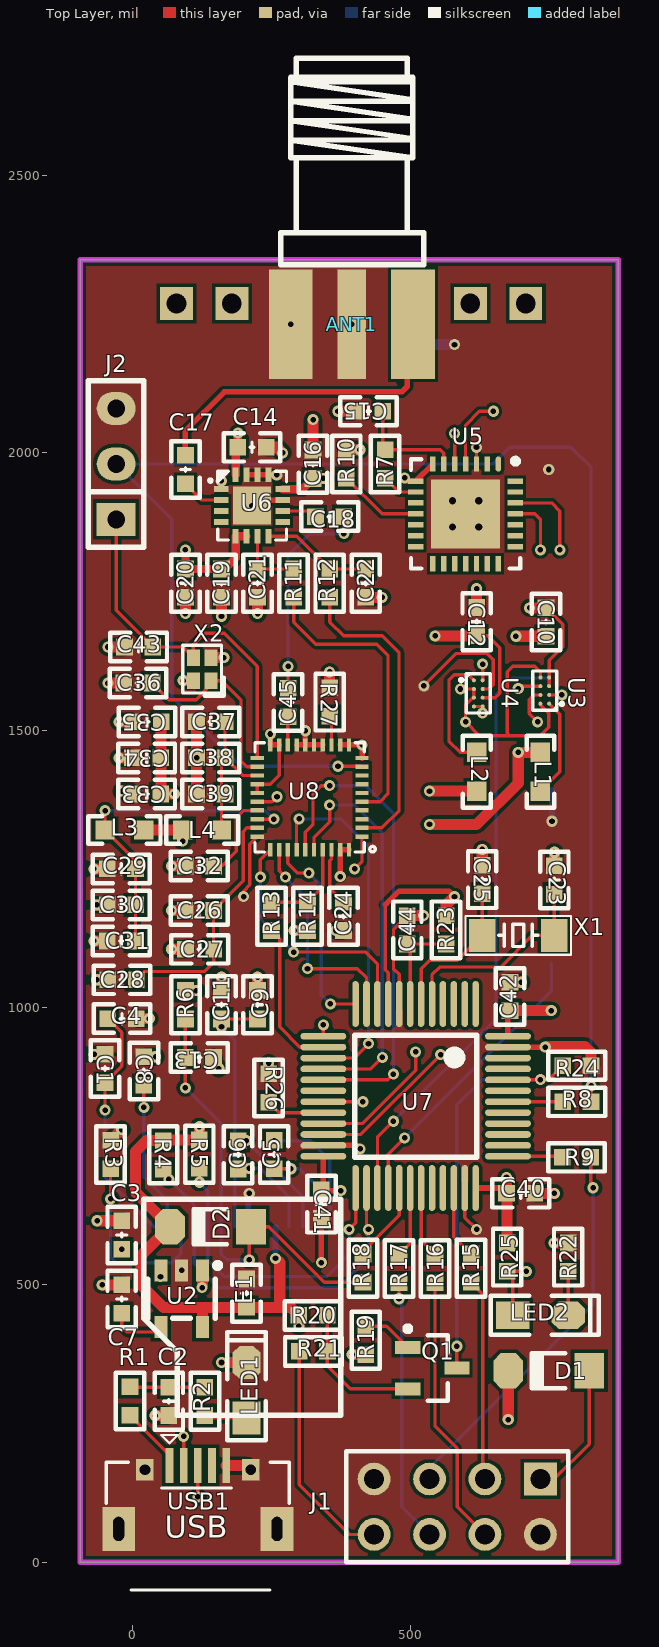
[diagram p0: Top Layer view]
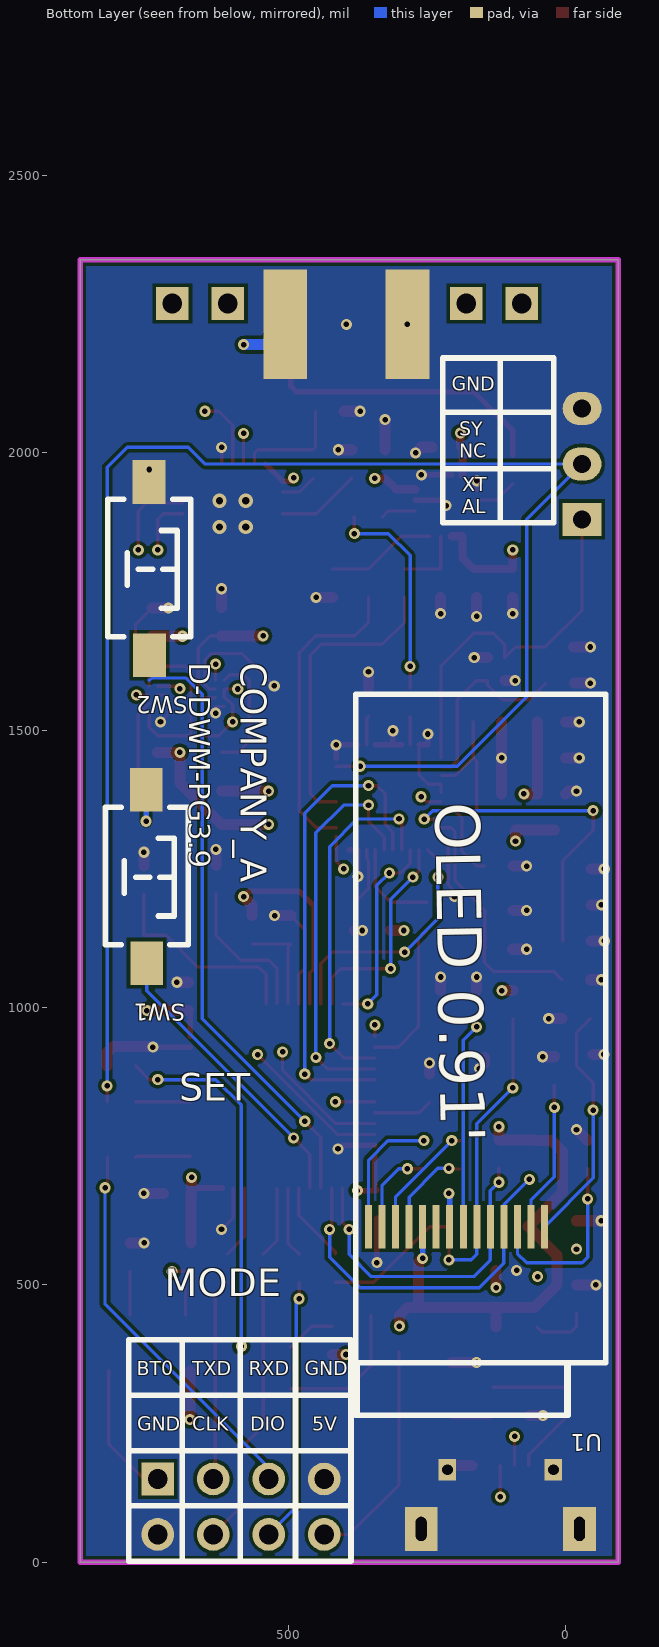
[diagram p1: Bottom Layer view, seen from below]
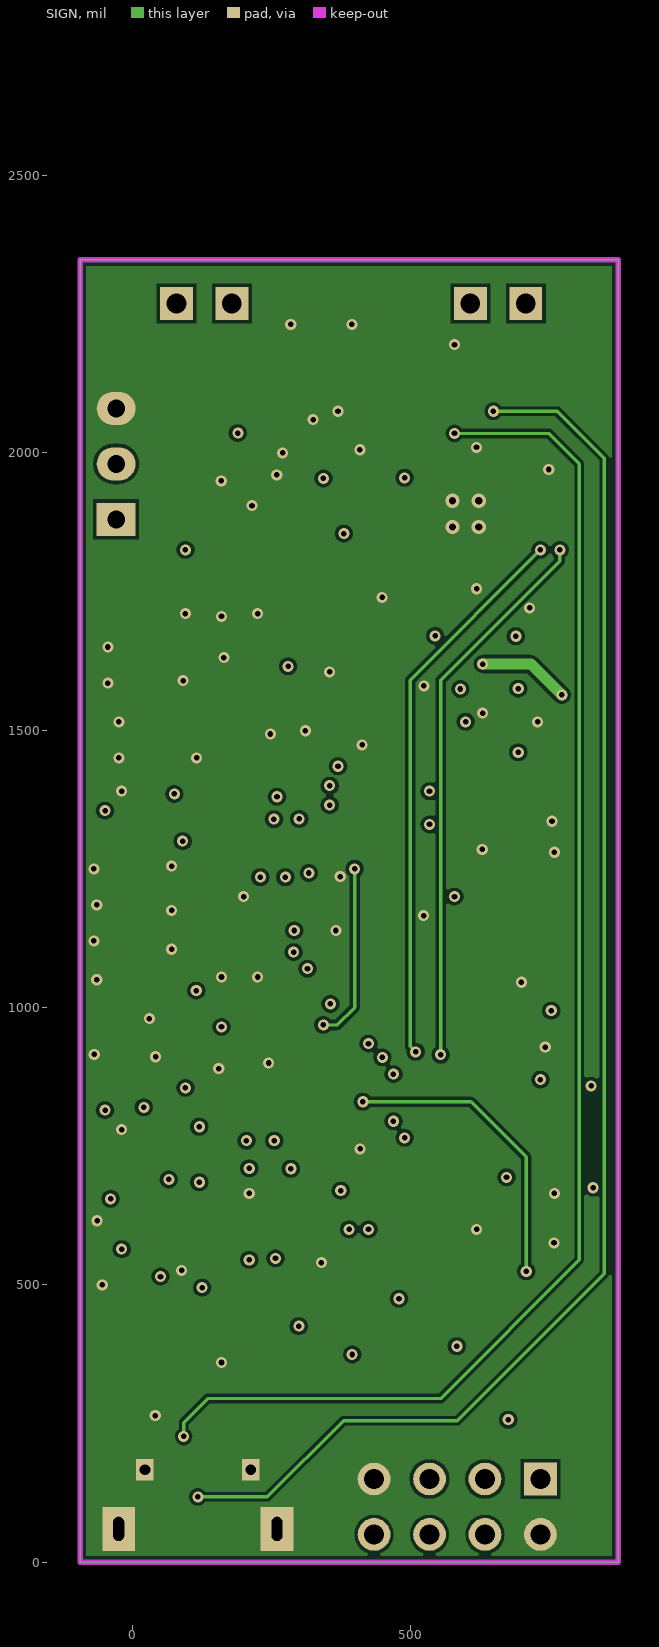
[diagram p2: SIGN]
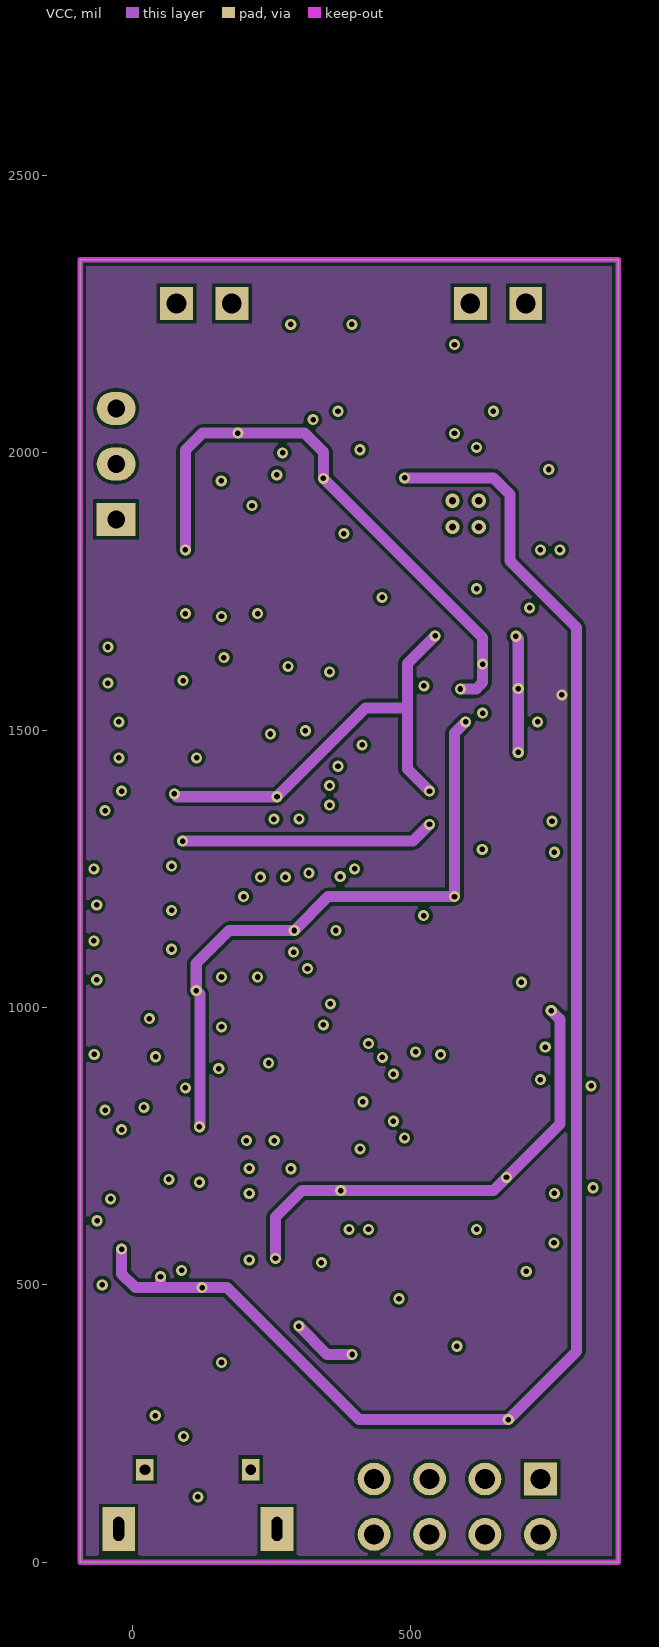
[diagram p3: VCC]
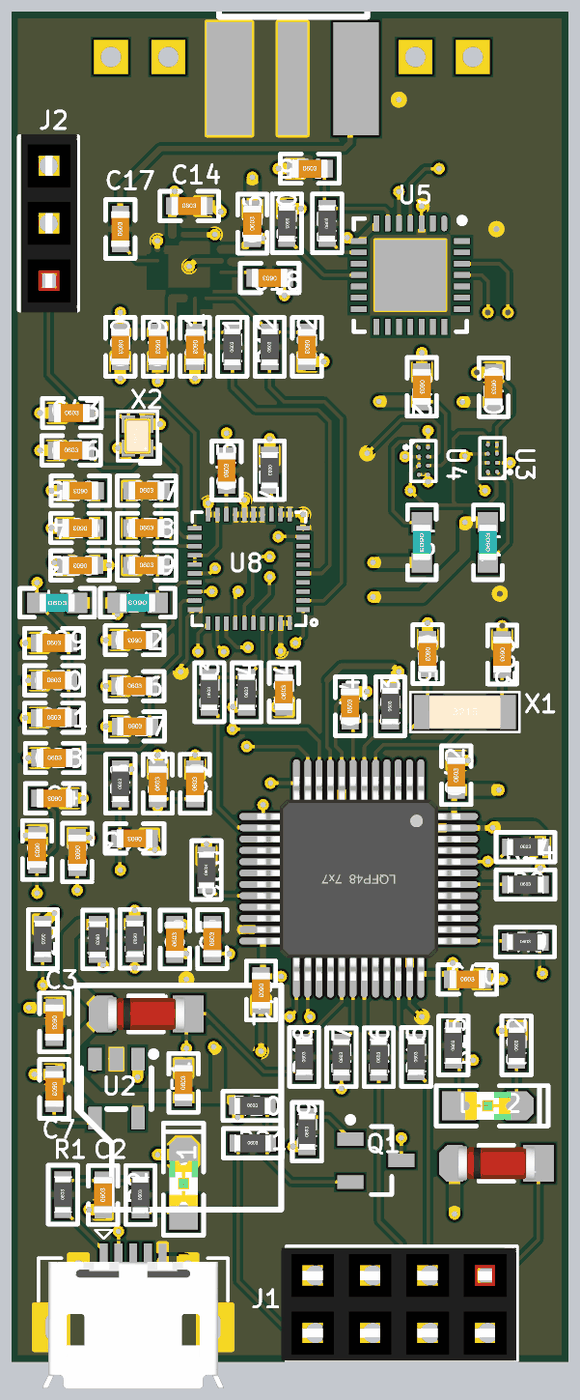
[diagram p4: 3D render of the assembled board from above, using the file's embedded part models]
# Altium PCB MISC85928.PcbDoc
Units mil, origin at the board's own origin, x right, y up, seen from the top; angles counter-clockwise.
Board outline 970 x 2348 mil, 4 copper layers (Top Layer, SIGN, VCC, Bottom Layer); 98 components, 80 nets, 373 pads, 153 vias.

## Layer stack, top to bottom (the 12.6 mil dielectric is the usual default, probably not edited)
Top Solder: solder mask 0.4, Solder Resist, Dk 3.5
Top Layer: signal copper 1.4
Dielectric1: core 12.6, FR-4, Dk 4.8
SIGN: signal copper 1.4
Dielectric3: core 12.6, FR-4, Dk 4.8
VCC: signal copper 1.4
Dielectric2: prepreg 12.6, FR-4, Dk 4.8
Bottom Layer: signal copper 1.4
Bottom Solder: solder mask 0.4, Solder Resist, Dk 3.5

## Board outline
-95,0 875,0 875,2348 -95,2348

## Design rules (kind name [scope] priority, off if disabled: settings)
Clearance [All] p1: gap=6 ignorepadtopadclearanceinfootprint=FALSE
MinimumSolderMaskSliver [All] p1: minsoldermaskwidth=0
PlaneConnect [All] p1: planeconnectstyle=Direct reliefexpansion=20 reliefentries=4 reliefconductorwidth=10 reliefairgap=10
PolygonConnect [All] p1: connectstyle=Direct reliefconductorwidth=10 reliefentries=4 polygonreliefangle="90 Angle" airgapwidth=10
RoutingVias [All] p1: holewidth=11.81 width=17.72 viastyle="Through Hole" minholewidth=11.81 minwidth=17.72 maxholewidth=11.81 maxwidth=17.72
SilkToSilkClearance [All] p1: silktosilkclearance=0
SilkToSolderMaskClearance SilkscreenOverComponentPads [IsPad] p1: minsilkscreentomaskgap=0 clearancetoexposedcopper=TRUE
SolderMaskExpansion [All] p1: expansion=4 istentingtop=FALSE
Width [All] p1: maxlimit=20 minlimit=5 preferedwidth=5
26 further rules are at their usual default settings.

## Components (designator, comment, footprint, x,y, rotation, side; value= is the part's Value field where it differs from the comment)
ANT1 "Partron" ÌìÏß×ù5p 395,2425 r90 top locked
C1 "100nF" "C 0603_L" -50,890 r270 top
C2 "100nF" "C 0603_L" 65,290 r90 top
C3 "10uF" "C 0603_L" -20,590 r270 top
C4 "4.7uF" "C 0603_L" -19.41,980 r180 top
C5 "1uF" "C 0603_L" 255,735 r90 top
C6 "1uF" "C 0603_L" 190,734.41 r90 top
C7 "100nF" "C 0603_L" -20,474.41 r270 top
C8 "2.2uF" "C 0603_L" 20,885.59 r270 top
C9 "100nF" "C 0603_L" 225,1005 r90 top
C10 "10uF" "C 0603_L" 745,1695 r270 top
C11 "4.7uF" "C 0603_L" 160,1005 r90 top
C12 "10uF" "C 0603_L" 620,1695.59 r270 top
C13 "4.7uF" "C 0603_L" 120,910 r180 top
C14 "1nF" "C 0603_L" 215,2010 r0 top
C15 "4.7uF" "C 0603_L" 425,2075 r0 top
C16 "1nF" "C 0603_L" 325,1979.41 r90 top
C17 "100pF" "C 0603_L" 95,1970 r90 top
C18 "100pF" "C 0603_L" 355,1885 r180 top
C19 "1nF" "C 0603_L" 160,1765 r270 top
C20 "1nF" "C 0603_L" 95,1765 r270 top
C21 "1nF" "C 0603_L" 225,1765 r270 top
C22 "1nF" "C 0603_L" 420,1765 r270 top
C23 "20pF" "C 0603_L" 760,1230 r270 top
C24 "100nF" "C 0603_L" 380,1164.41 r90 top
C25 "20pF" "C 0603_L" 630,1230.59 r270 top
C26 "2pF" "C 0603_L" 120,1175 r0 top
C27 "100nF" "C 0603_L" 120.59,1105 r0 top
C28 "22uF" "C 0603_L" -19.41,1050 r0 top
C29 "4.7nF" "C 0603_L" -20.59,1250 r0 top
C30 "100nF" "C 0603_L" -20.59,1185 r0 top
C31 "10uF" "C 0603_L" -20.59,1120 r0 top
C32 "220nF" "C 0603_L" 120,1255 r180 top
C33 "4.7nF" "C 0603_L" 25,1385 r180 top
C34 "100nF" "C 0603_L" 25,1450 r180 top
C35 "10uF" "C 0603_L" 25.59,1515 r180 top
C36 "8pF" "C 0603_L" 9.41,1585 r0 top
C37 "4.7nF" "C 0603_L" 140.59,1515 r0 top
C38 "100nF" "C 0603_L" 140.59,1450 r0 top
C39 "10uF" "C 0603_L" 140.59,1385 r0 top
C40 "100nF" "C 0603_L" 699.41,665 r0 top
C41 "100nF" "C 0603_L" 340,645.59 r270 top
C42 "100nF" "C 0603_L" 680,1020 r90 top
C43 "8pF" "C 0603_L" 10.59,1650 r0 top
C44 "100nF" "C 0603_L" 495,1140 r90 top
C45 "2pF" "C 0603_L" 280,1550 r90 top
D1 "SS34" "MINI_MELF (LL34)" 750,345 r180 top
D2 "1N4148" "MINI_MELF (LL34)" 140,605 r180 top
E1 "22uF/6.3V" "C 0603_L" 205,485 r90 top
J1 "Female HDR2X4" Fe-HDR2X4/2.54-S 735,150 r180 top locked
J2 "Female HDR1X3" Fe-HDR1X3/2.54-S -30,1880 r180 top
L1 "Inductor Iron" "L 0603" 735,1425 r90 top
L2 "Inductor Iron" "L 0603" 620,1425 r270 top
L3 "600R" "L 0603" -15,1320 r0 top
L4 "600R" "L 0603" 125,1320 r180 top
LED1 "Red" "LED 0805G" 205,310 r90 top
LED2 "Red" "LED 0805G" 735,445 r0 top
Q1 "S9012" SOT-23B_N 540,350 r0 top
R1 "B5R" "R 0603_L" -5,290.59 r90 top
R2 "470R" "R 0603_L" 130,290 r90 top
R3 "4.7K" "R 0603_L" -40,735 r270 top
R4 "4.7K" "R 0603_L" 55,734.41 r270 top
R5 "4.7K" "R 0603_L" 120,735.59 r270 top
R6 "4.7K" "R 0603_L" 95,1005 r90 top
R7 "4.7K" "R 0603_L" 455,1980 r90 top
R8 "0R" "R 0603_L" 800.59,830 r0 top
R9 "22R" "R 0603_L" 800,730 r0 top
R10 "10K" "R 0603_L" 385,1980 r270 top
R11 "0R" "R 0603_L" 290,1765 r90 top
R12 "0R" "R 0603_L" 355,1765 r90 top
R13 "100R" "R 0603_L" 250,1164.41 r90 top
R14 "DNF" "R 0603_L" 315,1164.41 r90 top
R15 "22R" "R 0603_L" 610,530 r90 top
R16 "22R" "R 0603_L" 545,529.41 r90 top
R17 "22R" "R 0603_L" 480,529.41 r90 top
R18 "22R" "R 0603_L" 415,530 r90 top
R19 "1K" "R 0603_L" 420,400 r90 top
R20 "1K" "R 0603_L" 325,445 r0 top
R21 "1K" "R 0603_L" 325.59,380 r0 top
R22 "470R" "R 0603_L" 785,550 r90 top
R23 "1K" "R 0603_L" 565,1140 r90 top
R24 "10K" "R 0603_L" 800.59,895 r0 top
R25 "10K" "R 0603_L" 675,550 r90 top
R26 "10K" "R 0603_L" 245,855 r90 top
R27 "49R9" "R 0603_L" 355,1550.59 r270 top
SW1 "3x6x5" "TSW SMD-3*6*2.5" 755,1235 r270 bottom
SW2 "3x6x5" "TSW SMD-3*6*2.5" 750,1790 r270 bottom
U1 "0.91-OLED" OLED0.91 152.67,914.72 r270 bottom locked
U2 "TPS736" SOT-23-5_L3.0-W1.7-P0.95-LS2.8-BR 90,475 r90 top
U3 "TPS62743YFPR" DSBGA-8_L1.6-W0.9-R2-C4-P0.40-BL 747.35,1571.38 r90 top
U4 "TPS62743YFPR" DSBGA-8_L1.6-W0.9-R2-C4-P0.40-BL 618.4,1566.38 r270 top
U5 "CP2102" CP2102 600,1890 r270 top
U6 "SW8112Q" QFN-16_L3.0-W3.0-P0.50-BL-EP1.7 16373.05,20632.78 r270 top
U7 "STM32F103C8T6" "LQFP48 7X7" 510,840 r180 top
U8 "DW3210" DW3210 325,1375 r180 top
USB1 "USB-5P" USB-MICRO_A 117.28,60 r0 top locked
X1 "16MHz" "OSC 3215-2P" 695,1130 r0 top
X2 "38.4MHZ" "OSC 1612-4P" 125,1610 r90 top

## Footprints (in the part's own frame and the unit in brackets; to place one, negate y for a bottom-side part, rotate by r counter-clockwise, add the part's x,y. Pads: shape width x height; smd on the part's side, far side on the other; paste and mask are expansions set on the pad)
"C 0603_L" [mil] "ÎÞ¼«ÐÔÌùÆ¬µçÈÝ"
  rect 30x30 smd: 1(-25.59,0) 2(25.59,0)
  silkscreen extent -51,-26 51,26, body extent -31,-16 31,16, height 32
CP2102 [mm]
  oval 0.7x0.25 smd paste+0 mask+0.051: 1(-2.28,1.5)
  rect 0.7x0.25 smd paste+0 mask+0.051: 2(-2.28,1) 3(-2.28,0.5) 4(-2.28,0) 5(-2.28,-0.5) 6(-2.28,-1) 7(-2.28,-1.5) 15(2.28,-1.5) 16(2.28,-1) 17(2.28,-0.5) 18(2.28,0) 19(2.28,0.5) 20(2.28,1) 21(2.28,1.5)
  rect 0.25x0.7 smd paste+0 mask+0.051: 8(-1.5,-2.28) 9(-1,-2.28) 10(-0.5,-2.28) 11(0,-2.28) 12(0.5,-2.28) 13(1,-2.28) 14(1.5,-2.28) 22(1.5,2.28) 23(1,2.28) 24(0.5,2.28) 25(0,2.28) 26(-0.5,2.28) 27(-1,2.28) 28(-1.5,2.28)
  rect 3.15x3.15 smd paste+0 mask+0.051: 29(0,0)
  silkscreen extent -2.54,-2.5 2.5,2.5
DSBGA-8_L1.6-W0.9-R2-C4-P0.40-BL [mm]
  round 0.184 smd paste+0 mask+0.051: A1(-0.6,-0.086) A2(-0.6,0.314) B1(-0.2,-0.086) B2(-0.2,0.314) C1(0.2,-0.086) C2(0.2,0.314) D1(0.6,-0.086) D2(0.6,0.314)
  silkscreen extent -0.9,-0.74 0.9,0.66
DW3210 [mm]
  rect 0.6x0.2 smd paste+0 mask+0.051: 1(-2.246,1.7) 2(-2.246,1.3) 3(-2.246,0.9) 4(-2.246,0.5) 5(-2.246,0.1) 6(-2.246,-0.3) 7(-2.246,-0.7) 8(-2.246,-1.1) 9(-2.246,-1.5) 10(-2.246,-1.9) 21(2.554,-1.9) 22(2.554,-1.5) 23(2.554,-1.1) 24(2.554,-0.7) 25(2.554,-0.3) 26(2.554,0.1) 27(2.554,0.5) 28(2.554,0.9) 29(2.554,1.3) 30(2.554,1.7)
  rect 0.2x0.6 smd paste+0 mask+0.051: 11(-1.646,-2.5) 12(-1.246,-2.5) 13(-0.846,-2.5) 14(-0.446,-2.5) 15(-0.046,-2.5) 16(0.354,-2.5) 17(0.754,-2.5) 18(1.154,-2.5) 19(1.554,-2.5) 20(1.954,-2.5) 31(1.954,2.3) 32(1.554,2.3) 33(1.154,2.3) 34(0.754,2.3) 35(0.354,2.3) 36(-0.046,2.3) 37(-0.446,2.3) 38(-0.846,2.3) 39(-1.246,2.3) 40(-1.646,2.3)
  silkscreen extent -2.85,-2.6 2.65,2.4
Fe-HDR1X3/2.54-S [mil]
  rect 70x60 hole 32: 1(0,0)
  oval 70x60 hole 32: 2(0,-100) 3(0,-200)
  silkscreen extent -50,-250 50,50, body extent -50,-255 48,55, height 335
Fe-HDR2X4/2.54-S [mm] "Connector; Header; 4x2 Position"
  rect 1.5x1.5 hole 0.9: 1(0,0)
  round 1.5 hole 0.9: 2(0,2.54) 3(2.54,0) 4(2.54,2.54) 5(5.08,0) 6(5.08,2.54) 7(7.62,0) 8(7.62,2.54)
  silkscreen extent -1.27,-1.27 8.89,3.81, body extent -1.27,-1.23 9.14,3.77, height 8.5
"L 0603" [mil] "Ð¡¹¦ÂÊÌùÆ¬µç¸Ð"
  rect 35x35 smd: 1(-35,0) 2(35,0)
  silkscreen extent -65,-25 65,25, body extent -31,-16 31,16, height 31
"LED 0805G" [mil] "ÂÌÉ«0805LED"
  rect 60x50 smd: 1(-50,0)
  oct 60x50 smd: 2(50,0)
  silkscreen extent -90,-35 105,35, body extent -39,-25 39,25, height 32
"LQFP48 7X7" [mm]
  oval 0.3x2.1 smd: 1(-2.75,-4.227) 2(-2.25,-4.227) 3(-1.75,-4.227) 4(-1.25,-4.227) 5(-0.75,-4.227) 6(-0.25,-4.227) 7(0.25,-4.227) 8(0.75,-4.227) 9(1.25,-4.227) 10(1.75,-4.227) 11(2.25,-4.227) 12(2.75,-4.227) 25(2.75,4.202) 26(2.25,4.202) 27(1.75,4.202) 28(1.25,4.202) 29(0.75,4.202) 30(0.25,4.202) 31(-0.25,4.202) 32(-0.75,4.202) 33(-1.25,4.202) 34(-1.75,4.202) 35(-2.25,4.202) 36(-2.75,4.202)
  oval 2.1x0.3 smd: 13(4.227,-2.75) 14(4.227,-2.25) 15(4.227,-1.75) 16(4.227,-1.25) 17(4.227,-0.75) 18(4.227,-0.25) 19(4.227,0.25) 20(4.227,0.75) 21(4.227,1.25) 22(4.227,1.75) 23(4.227,2.25) 24(4.227,2.75) 37(-4.227,2.75) 38(-4.227,2.25) 39(-4.227,1.75) 40(-4.227,1.25) 41(-4.227,0.75) 42(-4.227,0.25) 43(-4.227,-0.25) 44(-4.227,-0.75) 45(-4.227,-1.25) 46(-4.227,-1.75) 47(-4.227,-2.25) 48(-4.227,-2.75)
  silkscreen extent -2.79,-2.79 2.79,2.79, body extent -4.51,-4.5 4.5,4.5, height 1.45
"MINI_MELF (LL34)" [mm] "1.5*3.4mm(Ö±¾¶£¬½Å¾à£©"
  rect 1.37x1.62 smd: 1(-1.855,0)
  oct 1.37x1.62 smd: 2(1.855,0)
  silkscreen extent -0.76,-0.8 0.78,0.8, body extent -1.7,-0.75 1.7,0.75, height 1.5
OLED0.91 [mm]
  rect 2x0.32 smd paste+0 mask+0.051: 1(7.867,-5.139) 2(7.867,-4.519) 3(7.867,-3.899) 4(7.867,-3.279) 5(7.867,-2.659) 6(7.867,-2.039) 7(7.867,-1.419) 8(7.867,-0.799) 9(7.867,-0.179) 10(7.867,0.441) 11(7.867,1.061) 12(7.867,1.681) 13(7.867,2.301) 14(7.867,2.921)
  silkscreen extent -16.51,-5.72 16.51,5.71
"OSC 1612-4P" [mm] "1.6*1.2*0.35mm£¨³¤¿í¸ß£©"
  rect 0.75x0.6 smd: 1(-0.525,-0.4) 2(0.525,-0.4) 3(0.525,0.4) 4(-0.525,0.4)
  silkscreen extent -1.22,-0.99 1.09,0.89, body extent -0.8,-0.6 0.8,0.6, height 0.35
"OSC 3215-2P" [mm] "3.2*1.5*0.6mm(³¤¿í¸ß)"
  rect 1.2x1.5 smd: 1(-1.65,0) 2(1.65,0)
  silkscreen extent -2.41,-0.89 2.41,0.89, body extent -1.6,-0.75 1.6,0.75, height 0.61
QFN-16_L3.0-W3.0-P0.50-BL-EP1.7 [mm]
  rect 0.28x0.665 smd paste-100 mask+0.051: 1(474.935,-411.822) 2(475.435,-411.822) 3(475.936,-411.822) 4(476.436,-411.822) 9(476.436,-409.007) 10(475.936,-409.007) 11(475.435,-409.007) 12(474.935,-409.007)
  rect 0.665x0.28 smd paste-100 mask+0.051: 5(477.093,-411.165) 6(477.093,-410.665) 7(477.093,-410.165) 8(477.093,-409.665) 13(474.278,-409.665) 14(474.278,-410.165) 15(474.278,-410.665) 16(474.278,-411.165)
  rect 1.75x1.75 smd paste-100 mask+0.051: 17(475.685,-410.415)
  silkscreen extent 474.11,-412.39 477.26,-408.84
"R 0603_L" [mil] "1/10WÌùÆ¬µç×è"
  rect 30x30 smd: 1(-25.59,0) 2(25.59,0)
  silkscreen extent -51,-26 51,26, body extent -31,-16 32,16, height 16
SOT-23-5_L3.0-W1.7-P0.95-LS2.8-BR [mm]
  rect 1x0.6 smd paste+0 mask+0.051: 1(1.3,-0.899) 2(1.3,0.051) 3(1.3,1) 4(-1.3,1) 5(-1.3,-0.899)
  silkscreen extent -0.9,-1.73 1.65,1.6
SOT-23B_N [mm] "SOT23, 3-Leads, Body 2.9x1.3mm, Pitch 0.95mm, Lead Span 2.4mm, IPC Medium Density"
  rect 1.15x0.6 smd: 1(-1.125,0.95) 2(-1.125,-0.95) 3(1.125,0)
  silkscreen extent -1.25,-1.5 0.7,1.92, body extent -0.7,-1.5 0.7,1.5, height 1.14
"TSW SMD-3*6*2.5" [mm] "3*6*2.5mm"
  rect 2x1.5 smd: 1(-3.996,-0.02) 2(3.937,0)
  silkscreen extent -3.21,-1.9 3.09,1.9, body extent -4,-1.88 4,1.62, height 2.59
USB-MICRO_A [mm] "microÐÍUSB £¬5.7*7.8*2.5mm"
  rect 0.35x1.6 smd: 1(-1.3,2.9) 2(-0.65,2.9) 3(0,2.9) 4(0.65,2.9) 5(1.3,2.9)
  rect 1.5x2 hole 0.5 slot 1.1 at 90 deg: 5(-3.625,0) 5(3.625,0)
  rect 0.8x1 hole 0.5: 5(-2.425,2.71) 5(2.425,2.71)
  silkscreen extent -4.19,-2.79 4.19,4.3, body extent -4,-2.71 4,2.89, height 2.8
ÌìÏß×ù5p [mm]
  rect 5x2 smd paste+0 mask+0.102: 1(-4.91,-2.8) 2(-4.91,2.8)
  rect 5x2 smd far side paste+0 mask+0.102: 3(-4.91,2.8) 4(-4.91,-2.8)
  rect 5x1.3 smd paste+0 mask+0.102: 5(-4.91,0)
  silkscreen extent -2.18,-3.3 7.28,3.25

## Part data
C1 C2 C3 C4 C5 C6 C7 C8 C9 C10 C11 C12 C13 C14 C15 C16 C17 C18 C19 C20 C21 C22 C23 C24 C25 C26 C27 C28 C29 C30 C31 C32 C33 C34 C35 C36 C37 C38 C39 C40 C41 C42 C43 C44 C45: library part C, "Chip capacitor"
D1: library part 1N4148, "Switching diode"
D2: "Switching diode"
E1: library part CT, "Chip tantalum capacitor"
L1 L2: "Magnetic-Core Inductor"
L3 L4: library part L, "Low-power chip inductor"
LED1 LED2: library part LED-SMD, "Chip LED"
Q1: library part QNPN, "NPN Bipolar Transistor"
R1 R2 R3 R4 R5 R6 R7 R8 R9 R10 R11 R12 R13 R14 R15 R16 R17 R18 R19 R20 R21 R22 R23 R24 R25 R26 R27: library part R, "Chip resistor"
SW1 SW2: library part "TSW 3x6", "3x6 tact switch"
U2: library part TPS73633DBVR
U5: library part CP2102_1
USB1: "Micro USB female socket"
X1: library part XTAL-2P, "2-pin passive crystal"
X2: library part XTAL-ACT-4P, "4-pin active crystal oscillator"

## Free pads (board coordinates)
  rect 59.06x59.06 hole 35.43: 0(78.74,2269.26) 0(178.74,2269.26) 0(608.66,2269.26) 0(708.66,2269.26)

## Via types
v1: diameter 20, hole 10, Top Layer to Bottom Layer, 149 vias
v2: diameter 25.98, hole 12.99, Top Layer to Bottom Layer, tented both sides, 4 vias

## Nets (pads, with @x,y where several pads share a name; then routed paths per layer and width w, separated by ;. In a path a pad name is that pad's centre, name@x,y a point inside that pad or via, vN(x,y) a via of type N, cw(c..) or ccw(c..) an arc to the next point about the centre after c; other vN are vias at no path point)
1V5: C12.2 C33.1 C34.1 C35.1 L2.2 U4.C2 U8.26 | length 1326.2
  Top Layer w6: U8.26 251.07,1371.07 v1(260,1380) ; C12.2 640,1670 661.75,1648.25 661.75,1566.75 653.5,1558.5 U4.C2
  Top Layer w20: C35.1 50.59,1514.41 C34.1 C33.1 v1(75,1385) ; v1(535,1390) L2.2 ; v1(545,1670) C12.2
  VCC w20: v1(75,1385) 80,1380 v1(260,1380) 420,1540 495,1540 ; v1(535,1390) 495,1430 495,1540 ; v1(545,1670) 495,1620 495,1540
2V5: C10.2 L1.2 L3.2 L4.2 U3.C2 | length 1140.9
  Top Layer w6: v1(695,1575) 699.25,1579.25 U3.C2
  Top Layer w20: L3.2 L4.2 v1(90,1300) ; v1(535,1330) 620,1330 695,1405 v1(695,1460) L1.2 ; v1(690.59,1669.41) C10.2
  VCC w20: v1(90,1300) 505,1300 v1(535,1330) ; v1(690.59,1669.41) 695,1665 v1(695,1575) v1(695,1460)
3V3: C14.1 C16.1 C19.1 C20.1 C40.1 C41.1 C42.1 D2.2 E1.1 R4.1 R5.1 R6.2 R14.1 R19.1 R20.1 R23.2 R25.2 U1.5 U2.5 U3.A2 U3.B1 U3.D2 U4.A2 U4.B1 U4.C1 U6.5 U6.6 U6.12 U6.16 U7.9 U7.24 U7.36 U7.48 | length 6017.5
  Top Layer w6: 455,1185 455,1068.03 460.79,1062.24 U7.9 ; v1(590.75,1574.25) U4.B1 U4.C1 612.9,1558.5 600,1545.61 v1(600,1515) 625,1490 680,1490 ; U4.A2 v1(630.75,1619.25) ; U3.A2 735,1545.65 750,1530.65 750,1505 735,1490 680,1490 ; U3.D2 735,1605 725,1615 685,1615 675,1605 675,1495 680,1490 ; U3.B1 v1(773.5,1563.5)
  Top Layer w10: U7.24 343.58,674.76 C41.1 341.18,670 v1(375,670) ; 455,1185 480,1210 570,1210 v1(580,1200) ; U7.36 664.24,674.58 C40.1 ; U7.48 676.42,990.82 C42.1
  Top Layer w15: v1(95,1825) C20.1 C19.1 165.59,1790.59 185.47,1810.47 U6.5 U6.6 ; U6.16 185.47,2006.06 C14.1 v1(189.41,2035.59) ; U6.12 305.71,1934.53 C16.1 v1(343.82,1953.82)
  Top Layer w20: R6.2 v1(114.41,1030.59) ; v1(120,785) R5.1 56.18,761.18 R4.1 25,760 5,740 5,666.97 D2.2 15,553.03 15,500 55.49,459.51 144.51,459.51 144.41,459.41 ; U2.5 125.41,459.41 144.41,459.41 ; v1(257.36,547.64) 265,540 265,459.41 ; v1(291.18,1138.82) R14.1 ; v1(299.41,425.59) R20.1 285,459.41 265,459.41 ; v1(395.59,374.41) R19.1 ; R23.2 565,1185 v1(580,1200) ; v1(673.82,693.82) C40.1 675,663.82 R25.2 ; C42.1 v1(754.41,994.41) ; 144.41,459.41 E1.1 265,459.41
  VCC w20: v1(95,1825) 95,2005 125.59,2035.59 v1(189.41,2035.59) 309.41,2035.59 343.82,2001.18 v1(343.82,1953.82) 630.75,1666.89 v1(630.75,1619.25) 630.75,1585.75 619.25,1574.25 v1(590.75,1574.25) ; v1(120,785) 121,786 121,1024 v1(114.41,1030.59) 114.41,1079.41 173.82,1138.82 v1(291.18,1138.82) 352.36,1200 v1(580,1200) 580,1495 v1(600,1515) ; v1(257.36,547.64) 257.36,622.36 305,670 v1(375,670) 650,670 v1(673.82,693.82) 770,790 770,978.81 v1(754.41,994.41) ; v1(299.41,425.59) 350.59,374.41 v1(395.59,374.41)
  SIGN w20: v1(630.75,1619.25) 717.76,1619.25 v1(773.5,1563.5)
  Bottom Layer w10: v1(257.36,547.64) U1.5
5V: C3.2 D1.2 U2.1 U2.3 U5.7 U5.8 | length 3021.5
  Top Layer w10: v1(490,1955) 495.94,1949.06 U5.8 U5.7
  Top Layer w20: v1@125.41,500.41 U2.1 ; v1(676.97,256.97) D1.2
  VCC w20: v1(-20,564.41) -20,520 5,495 50,495 ; v1(50,515) 50,495 ; v1(490,1955) 650,1955 680,1925 680,1805 800.18,1684.82 800.18,380.18 v1(676.97,256.97) 408.03,256.97 170,495 v1(125,495) 50,495
BOOT0: Q1.3 R24.1 U7.44 | length 753.1
  Top Layer w6: Q1.3 v1(584.29,389.29) ; U7.44 676.89,870 v1(735,870) 750,870 R24.1
  Bottom Layer w6: v1(584.29,389.29) 584.29,824.29 630,870 v1(735,870)
BOOT1: R26.1 U7.20 | length 106.4
  Top Layer w6: R26.1 263.94,810.47 U7.20
DOWNLOAD: J1.8 R21.1 | length 412.3
  Top Layer w6: R21.1 300,140 390,50 J1.8
EXTON: U7.10 U8.31 | length 454.1
  Top Layer w6: v1(230,1235) 230,1266.39 U8.31 ; v1@285,1100 v1(290,1100) 420,1100 441.1,1078.9 U7.10
  Bottom Layer w6: v1(230,1235) 230,1160 v1(290,1100)
GND: ANT1.2 ANT1.3 ANT1.4 ANT1.5 C1.1 C2.1 C3.1 C4.1 C7.1 C8.1 C9.2 C10.1 C11.2 C12.1 C13.1 C14.2 C15.1 C16.2 C19.2 C20.2 C21.2 C22.2 C23.1 C24.1 C25.1 C26.1 C27.1 C28.1 C29.1 C30.1 C31.1 C32.2 C33.2 C34.2 C35.2 C36.1 C37.1 C38.1 C39.1 C40.2 C41.2 C42.2 C43.1 C44.2 E1.2 J1.2 J1.7 J2.3 LED1.2 R3.1 R10.1 R22.2 R24.2 R26.2 R27.1 SW1.1 SW2.1 U1.7 U2.2 U3.B2 U3.C1 U3.D1 U4.B2 U4.D1 U4.D2 U5.3 U5.29 U6.1 U6.11 U6.13 U6.14 U6.15 U6.17 U7.8 U7.23 U7.35 U7.47 U8.10 U8.11 U8.12 U8.14 U8.15 U8.16 U8.17 U8.19 U8.20 U8.24 U8.25 U8.30 U8.39 U8.40 USB1.5 X2.2 X2.4 | length 3279.1
  Top Layer w6: v1(200,1200) 200,1210 211,1221 211,1294.63 U8.30 ; U8.25 U8.24 247.57,1402.57 263.82,1418.82 U8.19 ; U7.8 480.47,1059.53 470,1070 470,1140.58 C44.2 ; v1(525,1580) 583.25,1638.25 638.62,1638.25 649.75,1627.12 649.75,1581.72 642.28,1574.25 U4.B2 ; U7.35 598.58,621.42 v1(620,600) ; U4.D1 U4.D2 v1(630.75,1530.75) ; U5.3 v1(619.68,2009.68) ; v1(730,1515) 715,1530 715,1555 723.5,1563.5 U3.B2 ; C10.1 775,1690.59 775,1650 750.75,1625.75 U3.D1 U3.C1
  Top Layer w10: U6.1 v1(159.59,1949.59) ; U6.15 U6.14 U6.13 v1(259.59,1960.41) ; v1(215,1905) 224.84,1914.84 U6.11 ; v1(248.07,1493.07) U8.20 U8.19 ; U8.17 U8.16 ; v1(311.06,1498.94) U8.16 ; v1(340,540) C41.2 ; U8.14 U8.15 U8.16 ; U7.23 403.58,751.42 v1(410,745) ; v1(374.06,1235.94) U8.39 U8.40 ; U8.12 U8.11 v1(413.43,1473.43) U8.10 ; U7.47 v1(743.58,928.58) v1@745,930
  Top Layer w20: v1(-70,1120) C31.1 ; v1(-70,1250) C29.1 ; v1(-69.41,915.59) C1.1 ; v1(-65,1050) C28.1 ; v1(-65,1185) C30.1 ; v1(-64.41,615.59) C3.1 ; v1(-55,500) C7.1 ; v1(-45,1585) C36.1 ; v1(-45,1650) C43.1 ; R3.1 -39.41,760.59 v1(-20,780) ; v1(-25,1450) C34.2 ; v1(-25,1515) C35.2 ; v1(-20,1390) -5.58,1390 C33.2 ; C4.1 v1(30,980) ; C8.1 v1(41.18,911.18) ; v1(40.59,264.41) C2.1 ; v1(70,1105) C27.1 ; v1(70,1175) C26.1 ; v1(70,1255) C32.2 ; v1(90.67,1589.33) X2.4 ; v1(95,1710) C20.2 ; C39.1 v1(115,1450) C37.1 ; X2.2 v1(164.33,1630.67) ; C13.1 145.59,899.41 v1(155,890) ; v1(160,360) LED1.2 ; C11.2 v1(160,1055) ; v1(160,1705) C19.2 ; USB1.5@168.46,174.17 205.28,174.17 USB1.5@212.76,166.69 ; C9.2 v1(225,1055) ; v1(225,1710) C21.2 ; C14.2 260,2010 v1(270,2000) ; R26.2 v1(245,900) ; C16.2 v1(325,2060) ; R27.1 v1(355,1605) ; v1(366.18,1138.82) C24.1 ; v1(370,2075) C15.1 ; R10.1 v1(409.41,2005.59) ; C22.2 v1(449.41,1739.41) ; C44.2 v1(524.41,1165.59) ; C12.1 v1(620,1755) ; C25.1 v1(630,1285) ; C42.2 v1(700.59,1045.59) ; v1(715.59,1720.59) C10.1 ; C40.2 v1(760,665) ; v1@745,930 815,930 826.18,918.82 R24.2 ; v1(759.41,575.59) R22.2 ; C23.1 v1(760,1280)
  Bottom Layer w10: U1.7 v1@208.54,663.54 ; v1(755.79,1335.79) SW1.1
  Bottom Layer w20: ANT1.4 541.95,2195 v1(580,2195)
  other v1: 88.01,526.19 210,665 750,1970 284.76,2231.71 395,2231.71
  other v2: 576.38,1866.38 623.62,1866.38 576.38,1913.62 623.62,1913.62
GPIO5: R11.1 U8.5 | length 541.6
  Top Layer w6: R11.1 290,1695 330,1655 440,1655 460,1635 460,1385 446.07,1371.07 U8.5
GPIO6: R12.1 U8.2 | length 556.7
  Top Layer w6: R12.1 355,1695 380,1670 450,1670 480,1640 480,1355 448.83,1323.83 U8.2
IRQN: U7.13 U8.1 | length 403.4
  Top Layer w6: U7.13 v1(343.58,968.58) ; v1(400,1250) 413.42,1263.42 U8.1
  SIGN w6: v1(343.58,968.58) 368.58,968.58 400,1000 v1(400,1250)
KEY1: SW1.2 U7.28 | length 527.3
  Top Layer w6: U7.28 460.79,735.79 v1(490,765)
  Bottom Layer w6: v1(490,765) 755,1030 SW1.2
KEY2: SW2.2 U7.27 | length 1087.7
  Top Layer w6: U7.27 441.1,766.1 v1(470,795)
  Bottom Layer w6: v1(470,795) 655,980 655,1565 684,1594 746,1594 750,1590
LED: LED2.1 R25.1 U7.19 | length 732
  Top Layer w6: U7.19 v1(414.84,830.16) ; LED2.1 685,514.41 R25.1 v1(709.41,524.41) v1@710,525
  SIGN w6: v1(414.84,830.16) 609.84,830.16 709.41,730.59 v1(709.41,524.41)
NetANT1_1: ANT1.1 C17.2 | length 593.5
  Top Layer w10: C17.2 95,2040 165,2110 485,2110 495,2120 495,2221.47 ANT1.1
NetC1_2: C1.2 C4.2 U1.14 | length 439.1
  Top Layer w6: v1(-50,815) C1.2 -20,894.42 -20,955 C4.2
  Bottom Layer w6: v1@-50,820 v1(-50,815) -50,692.68 U1.14
NetC2_2: C2.2 R1.2 R2.2 | length 135.2
  Top Layer w6: R1.2 -4.41,315.59 C2.2 R2.2
NetC5_1: C5.1 U1.2 | length 162.4
  Top Layer w6: C5.1 v1(285,709.41)
  Bottom Layer w6: v1(285,709.41) 300.59,709.41 330.59,679.41 U1.2
NetC5_2: C5.2 U1.1 | length 234.5
  Bottom Layer w6: v1(255,760) 320,760 355,725 U1.1
NetC6_1: C6.1 U1.4 | length 166.9
  Top Layer w6: C6.1 208.82,708.82 v1(210,710)
  Bottom Layer w6: v1(210,710) 230,710 281.77,658.23 U1.4
NetC6_2: C6.2 U1.3 | length 211.9
  Top Layer w6: C6.2 v1(205,760)
  Bottom Layer w6: v1(205,760) 306.18,658.82 U1.3
NetC7_2: C7.2 U2.4 | length 102.2
  Top Layer w6: C7.2 -20,425 -10,415 41.79,415 U2.4
NetC8_2: C8.2 U1.13 | length 272.4
  Top Layer w6: v1(20,820) C8.2
  Bottom Layer w6: v1(20,820) 20,695 62.09,652.91 U1.13
NetC9_1: C9.1 C11.1 U1.8 | length 435
  Top Layer w6: C11.1 C9.1
  Bottom Layer w6: v1(160,965) 184.13,940.87 U1.8
NetC15_2: C15.2 R7.2 U5.6 | length 199.1
  Top Layer w6: C15.2 450.59,2010 R7.2 554.41,2005.59 560.63,1999.37 U5.6
NetC17_1: C17.1 U6.2 | length 76.8
  Top Layer w6: C17.1 124.57,1914.84 U6.2
NetC18_2: C18.2 U6.10 | length 63.2
  Top Layer w6: U6.10 319.26,1895.16 C18.2
NetC21_1: C21.1 R11.2 U6.7 | length 124.1
  Top Layer w6: U6.7 224.84,1790.75 C21.1 R11.2
NetC22_1: C22.1 R12.2 U6.8 | length 199.9
  Top Layer w6: U6.8 296,1849.59 R12.2 C22.1
NetC23_2: C23.2 U7.5 X1.2 | length 377.2
  Top Layer w6: U7.5 539.53,1059.53 553,1073 663,1073 720,1130 X1.2 C23.2 C23.2
NetC24_2: C24.2 U8.38 | length 106.2
  Top Layer w6: U8.38 358.31,1268.31 355,1265 355,1215 C24.2
NetC25_2: C25.2 U7.6 X1.1 | length 273.6
  Top Layer w6: U7.6 519.84,1069.84 535,1085 585.04,1085 X1.1 C25.2 C25.2
NetC26_2: C26.2 C27.2 C28.2 U8.29 | length 439.4
  Top Layer w6: C28.2 21.18,1065 130,1065 146.18,1081.18 C27.2 145.59,1105.59 C26.2 199,1228.41 199,1317 205.83,1323.83 U8.29
NetC29_2: C29.2 C30.2 C31.2 L3.1 U8.28 | length 598.9
  Top Layer w6: v1(-50,1355) L3.1 5,1265 C29.2 C30.2 C31.2 ; U8.28 v1(254.58,1339.58)
  Bottom Layer w6: v1(-50,1355) 239.15,1355 v1(254.58,1339.58)
NetC37_2: C37.2 C38.2 C39.2 L4.1 U8.23 | length 269
  Top Layer w6: L4.1 160,1443.82 C38.2 ; C37.2 C38.2 ; U8.23 197.86,1418.32 C38.2
NetC45_1: C45.1 U8.18 | length 51.2
  Top Layer w6: U8.18 279.57,1523.97 C45.1
NetD1_1: D1.1 J1.1 | length 246.1
  Top Layer w6: J1.1 760,150 823.03,213.03 D1.1
NetL1_1: L1.1 U3.A1 | length 180.2
  Top Layer w6: L1.1 770,1425 770,1528.5 U3.A1
NetL2_1: L2.1 U4.A1 | length 221.6
  Top Layer w6: U4.A1 605,1600 580,1600 570,1590 570,1480 590,1460 L2.1
NetLED1_1: LED1.1 R2.1 | length 76.8
  Top Layer w6: R2.1 134.41,260 LED1.1
NetLED2_2: LED2.2 R22.1 | length 79.4
  Top Layer w6: LED2.2 R22.1
NetQ1_1: Q1.1 R19.2 | length 91.5
  Top Layer w6: R19.2 457.52,425.59 Q1.1
NetQ1_2: Q1.2 R20.2 R21.2 | length 253
  Top Layer w6: R20.2 350.59,354.41 392.4,312.6 Q1.2
NetR1_1: R1.1 USB1.1 | length 120.3
  Top Layer w6: R1.1 66.1,193.9 USB1.1
NetR3_2: R3.2 U1.12 | length 345.4
  Top Layer w6: v1(-40,655) R3.2
  Bottom Layer w6: v1(-40,655) -40,550 -30,540 70,540 86.5,556.5 U1.12
NetR7_1: R7.1 U5.9 | length 65.6
  Top Layer w6: R7.1 480.04,1929.37 U5.9
NetR8_1: R8.1 U7.42 | length 98.6
  Top Layer w6: U7.42 774.84,830.16 R8.1
NetR9_1: R9.1 U7.37 | length 98.7
  Top Layer w6: U7.37 772.67,731.73 R9.1
NetR10_2: R10.2 U5.11 | length 151.9
  Top Layer w6: R10.2 449.41,1890 U5.11
NetR13_2: R13.2 R14.2 U8.37 | length 170.9
  Top Layer w6: R13.2 R14.2 342.56,1217.56 U8.37
NetR15_2: R15.2 U7.34 | length 131.9
  Top Layer w6: U7.34 578.9,586.69 R15.2
NetR16_2: R16.2 U7.31 | length 130
  Top Layer w6: U7.31 519.84,580.16 R16.2
NetR17_2: R17.2 U7.30 | length 127.9
  Top Layer w6: R17.2 500.16,575.16 U7.30
NetR18_2: R18.2 U7.29 | length 146.1
  Top Layer w6: R18.2 415,560 480.47,625.47 U7.29
NetR27_2: R27.2 U8.13 | length 52.9
  Top Layer w6: R27.2 358.31,1521.69 U8.13
NRST: C44.1 R23.1 U7.7 | length 180.1
  Top Layer w6: U7.7 500.16,1109.25 C44.1 R23.1
OLED_REST: C13.2 D2.1 R6.1 R18.1 U1.9 | length 810.9
  Top Layer w6: v1(95,855) 94.41,855.59 C13.2 94.41,978.82 R6.1 ; v1(210,545) 210,601.97 D2.1 245,605 345.59,504.41 R18.1
  Bottom Layer w6: v1(95,855) 159.73,790.27 U1.9 159.73,555.27 170,545 v1(210,545)
PC13: U7.2
RF_IN: C18.1 C45.2 | length 386.9
  Top Layer w6: C45.2 v1(280,1615) ; v1(380.59,1854.41) C18.1
  Bottom Layer w6: v1(280,1615) 280,1815 319.41,1854.41 v1(380.59,1854.41)
RSTN: U7.12 U8.33 | length 366.9
  Top Layer w6: U8.33 279.57,1260.43 297.5,1242.5 v1(317.5,1242.5) ; v1(356.42,1006.42) U7.12
  Bottom Layer w6: v1(317.5,1242.5) 340,1220 340,1022.83 v1(356.42,1006.42)
RXD1: J1.4 R16.1 | length 491.1
  Top Layer w6: R16.1 545,245 585,205 585,100 J1.4
RXD3: U5.26 U7.22 | length 1426.4
  Top Layer w6: U7.22 411.1,771.1 v1(555,915) ; U5.26 755.32,1909.68 770,1895 v1(770,1825)
  SIGN w6: v1(555,915) 555,1590 770,1805 v1(770,1825)
SCL: R5.2 U1.10 U7.25 | length 579.7
  Top Layer w6: v1(120,685) R5.2 ; v1(390,600) 401.73,611.73 U7.25
  Bottom Layer w6: v1(120,685) 135.32,669.69 U1.10 135.32,544.69 165,515 350,515 390,555 v1(390,600)
SDA: R4.2 U1.11 U7.26 | length 658.2
  Top Layer w6: v1@421.42,591.42 U7.26
  Bottom Layer w6: v1(65,690) 110.91,644.09 U1.11 110.91,539.09 155,495 370,495 425,550 v1(425,600)
SPICLK: U7.15 U8.34 | length 650.4
  Top Layer w6: U8.34 295.31,1335.31 v1(300,1340) ; U7.15 398.9,908.9 v1(425,935)
  Bottom Layer w6: v1(300,1340) 375,1340 425,1290 v1(425,935)
SPICSN: R13.1 U7.14 | length 273.7
  Top Layer w6: R13.1 265,1123.82 265,965 301.42,928.58 U7.14
SPIMISO: U7.16 U8.36 | length 728
  Top Layer w6: U8.36 326.81,1306.81 355,1335 v1(355,1365) ; U7.16 429.21,889.21 v1(450,910)
  Bottom Layer w6: v1(355,1365) 400,1365 450,1315 v1(450,910)
SPIMOSI: U7.17 U8.35 | length 879
  Top Layer w6: U8.35 311.06,1316.06 325,1330 325,1385 340,1400 v1(355,1400) ; U7.17 459.53,869.53 v1(470,880)
  Bottom Layer w6: v1(355,1400) 420,1400 470,1350 v1(470,880)
SWCLK: J1.5 R9.2 | length 704
  Top Layer w6: R9.2 825.59,679.41 v1(830,675)
  Bottom Layer w6: J1.5 535,170 830,465 v1(830,675)
SWDIO: J1.3 R15.1 | length 364.8
  Top Layer w6: R15.1 631,483.41 631,154 J1.3
SYNC: J2.2 R8.2 U8.9 | length 2884.4
  Top Layer w6: v1(370,1435) 412.49,1435 U8.9 ; R8.2 v1(826.18,858.82)
  Bottom Layer w6: v1(370,1435) 195,1435 70,1560 70,1880 J2.2 650,1980 680,2010 790,2010 826.18,1973.82 v1(826.18,858.82)
TXD1: J1.6 R17.1 | length 476.6
  Top Layer w6: v1(480,475) R17.1
  Bottom Layer w6: v1(480,475) 485,470 485,100 J1.6
TXD3: U5.25 U7.21 | length 1350.2
  Top Layer w6: U7.21 413.82,790.79 510,886.97 v1(510,920) ; U5.25 725,1890 735,1880 v1(735,1825)
  SIGN w6: v1(510,920) 500,930 500,1590 v1(735,1825)
USB_D+: U5.4 USB1.3 | length 2791.6
  Top Layer w6: v1(117.28,117.72) USB1.3 ; U5.4 600,2050 625,2075 v1(650,2075)
  SIGN w6: v1(117.28,117.72) 242.72,117.72 380,255 585,255 850,520 850,1990 765,2075 v1(650,2075)
USB_D-: U5.5 USB1.2 | length 2650.5
  Top Layer w6: USB1.2 v1(91.69,226.69) ; v1(580,2035) 580.31,2034.69 U5.5
  SIGN w6: v1(91.69,226.69) 91.69,251.69 135,295 555,295 805,545 805,1980 750,2035 v1(580,2035)
VDDHV_TX: C32.1 U8.27 | length 155.7
  Top Layer w6: C32.1 160,1255 186.5,1281.5 186.5,1341.23 186.36,1341.36 200.32,1355.32 U8.27
WAKEUP: U7.11 U8.32 | length 396
  Top Layer w6: U8.32 263.82,1246.18 v1(275,1235) ; v1(315,1070) 405,1070 421.42,1053.58 U7.11
  Bottom Layer w6: v1(275,1235) 315,1195 v1(315,1070)
XTAL1: C43.2 J2.1 U8.21 X2.3 | length 676.2
  Top Layer w6: J2.1 -30,1716.18 C43.2 89.92,1650 X2.3 109.25,1654.25 130,1675 165,1675 224.45,1615.55 U8.21
XTAL2: C36.2 U8.22 X2.1 | length 349.4
  Top Layer w6: C36.2 65,1555 114.22,1555 140.75,1581.52 X2.1 160.67,1589.33 195,1555 195,1445 205.94,1434.07 U8.22
pads on no net: U1.6 U5.1 U5.2 U5.10 U5.12 U5.13 U5.14 U5.15 U5.16 U5.17 U5.18 U5.19 U5.20 U5.21 U5.22 U5.23 U5.24 U5.27 U5.28 U6.3 U6.4 U6.9 U7.1 U7.3 U7.4 U7.18 U7.32 U7.33 U7.38 U7.39 U7.40 U7.41 U7.43 U7.45 U7.46 U8.3 U8.4 U8.6 U8.7 U8.8 USB1.4

## Polygon pours and split planes (outlines as drawn)
GND on SIGN "D" (solid, remove dead copper, pour order 2): -215,2395 970,2395 1020,2445 985,2410 985,-230 -220,-230 -330,-120
3V3 on VCC "D" (solid, remove dead copper, pour order 4): -210,2385 -195,2400 940,2400 940,-80 910,-50 -170,-50
GND on Top Layer "D" (solid, remove dead copper, pour order 6): -290,2400 925,2400 960,2435 915,2390 915,-95 -75,-95 -145,-165
GND on Bottom Layer "D" (solid, remove dead copper, pour order 8): -240,2370 -200,2410 930,2410 930,-145 905,-170 890,-155 -190,-155

## Keep-outs
Keep-Out Layer:
  the board outline again, w10

## Silkscreen, mask and mechanical layers (free items; w line width, h text height)
Bottom Overlay:
  lines w10: 20.8,2073 221.41,2073 ; 117.41,1875 117.41,1971.2 117.41,2171 ; 219.41,1874 20.8,1874 20.8,1971.2 ; 221.41,1874 221.41,1971.2 ; 386.59,300.99 787.2,300.99 ; 386.98,102.1 787.59,102.1 ; 486.59,1.31 486.59,201.1 486.59,397.9 ; 586.59,1.31 586.59,201.1 586.59,399.9 ; 690.59,1.31 690.59,201.1 690.59,399.1 ; 20.8,1971.2 20.8,2171 221.41,2171 221.41,1971.2 ; 20.8,1971.2 221.41,1971.2 ; 386.59,201.1 787.2,201.1 ; 386.59,201.1 386.59,400.9 787.2,400.9 787.2,201.1 ; 386.59,201.1 386.59,1.31 787.2,1.31 787.2,201.1
  text "GND" at 205,2112 h25
  text "SY" at 191,2031 h25
  text "NC" at 191,1991 h25
  text "XT" at 186,1931 h25
  text "AL" at 186,1891 h25
  text "COMPANY_A" at 600.2,1621.2 h80 r90
  text "D-DWM-PG3.9" at 691.2,1621.2 h65 r90
  text "SET" at 696.5,831.5 h50
  text "MODE" at 722.5,479.5 h50
  text "GND" at 469.59,337.1 h25
  text "RXD" at 570.59,337.1 h25
  text "TXD" at 672.59,337.1 h25
  text "BT0" at 772.59,337.1 h25
  text "5V" at 456.59,237.1 h25
  text "DIO" at 568.59,237.1 h25
  text "CLK" at 672.59,237.1 h25
  text "GND" at 771.59,237.1 h25